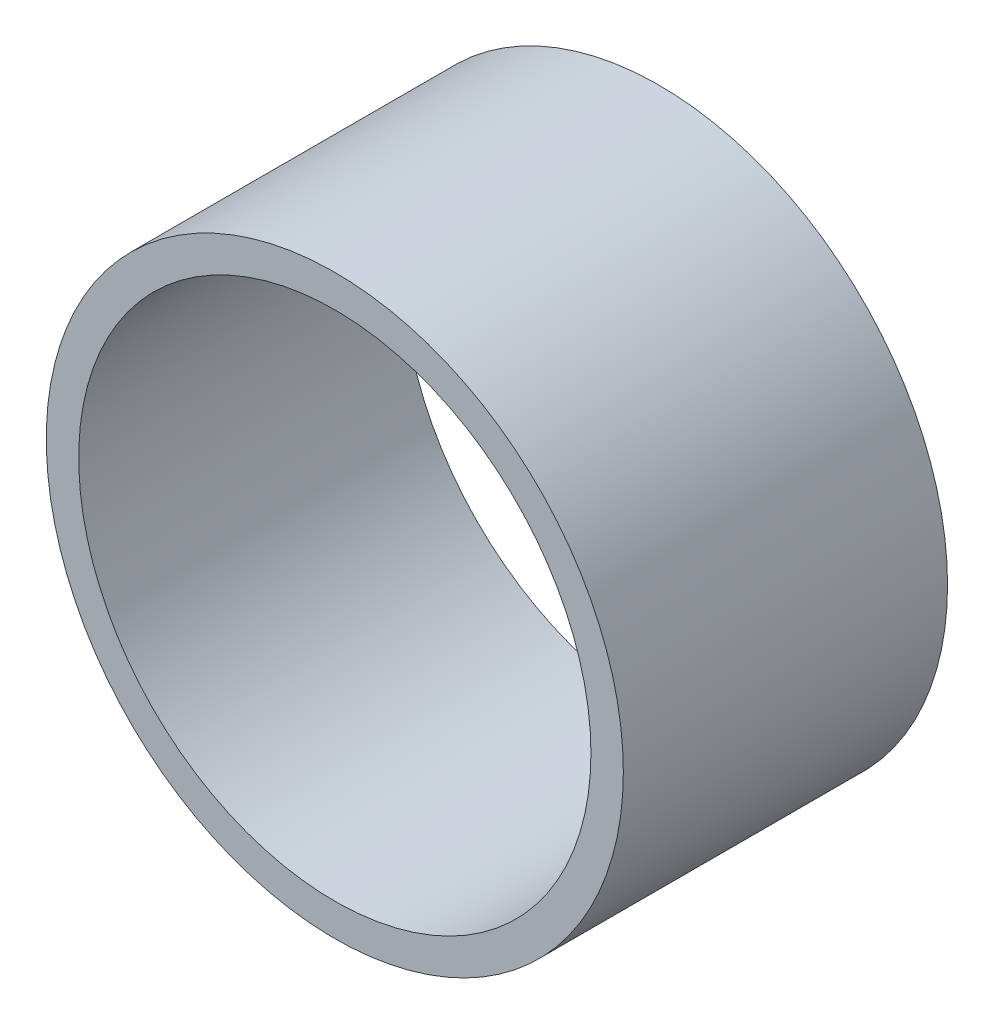
from build123d import *

# Parameters (mm, degrees)
SKETCH1_R           = 44.5
SKETCH1_R_2         = 39.5
BOSS_EXTRUDE1_DEPTH = 50


with BuildPart() as part:
    # Sketch1 → Boss-Extrude1 (new body)
    with BuildSketch(Plane.XY):
        Circle(SKETCH1_R)
        Circle(SKETCH1_R_2, mode=Mode.SUBTRACT)
    extrude(amount=BOSS_EXTRUDE1_DEPTH)


solid = part.part
